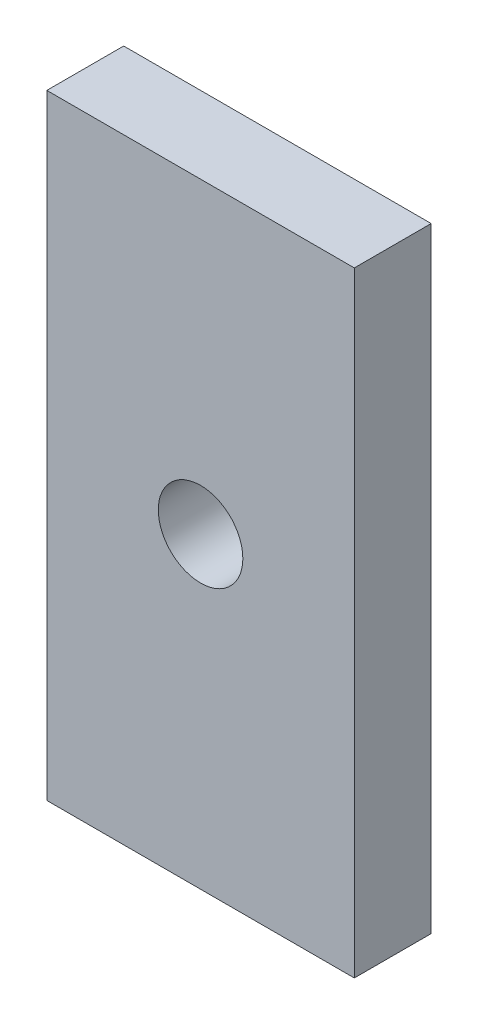
SolidWorks part; units mm, degrees
material "Q235"
ref_plane "Front Plane" through (0, 0, 0) normal (0, 0, 1) x (1, 0, 0)
ref_plane "Top Plane" through (0, 0, 0) normal (0, 1, 0) x (1, 0, 0)
ref_plane "Right Plane" through (0, 0, 0) normal (1, 0, 0) x (0, 0, -1)
sketch "Sketch1" plane through (0, 0, 0) normal (0, 0, 1) x (1, 0, 0)
  line L1 (0, 0) -> (40, 0)
  line L2 (0, 0) -> (0, 80)
  line L3 (0, 80) -> (40, 80)
  line L4 (40, 0) -> (40, 80)
  dimension "D1" = 40
  dimension "D2" = 80
extrude "Boss-Extrude1" add sketch "Sketch1" along normal blind 10
hole_wizard "Ø11.0 (11) Diameter Hole1" positions "Sketch2" profile "Sketch3" hole size "Ø11.0" standard "GB" end condition through all
sketch "Sketch2" plane through (0, 0, 10) normal (0, 0, 1) x (1, 0, 0)
  line L13 (20, 40) -> (0, 40) construction
  line L14 (0, 80) -> (0, 0) construction
  line L17 (20, 40) -> (20, 0) construction
  line L18 (0, 0) -> (40, 0) construction
  point P6 (20, 40)
sketch "Sketch3" plane through (20, 40, 10) normal (1, 0, 0) x (0, -1, 0)
  line L0 (0, 0) -> (0, 10)
  line L1 (0, 10) -> (5.5, 10)
  line L2 (5.5, 10) -> (5.5, 0)
  line L5 (5.5, 0) -> (0, 0)
  line L11 (0, -6.35) -> (0, 107.95) construction
  dimension "通孔孔直径" = 11
  dimension "通孔孔深度" = 10
